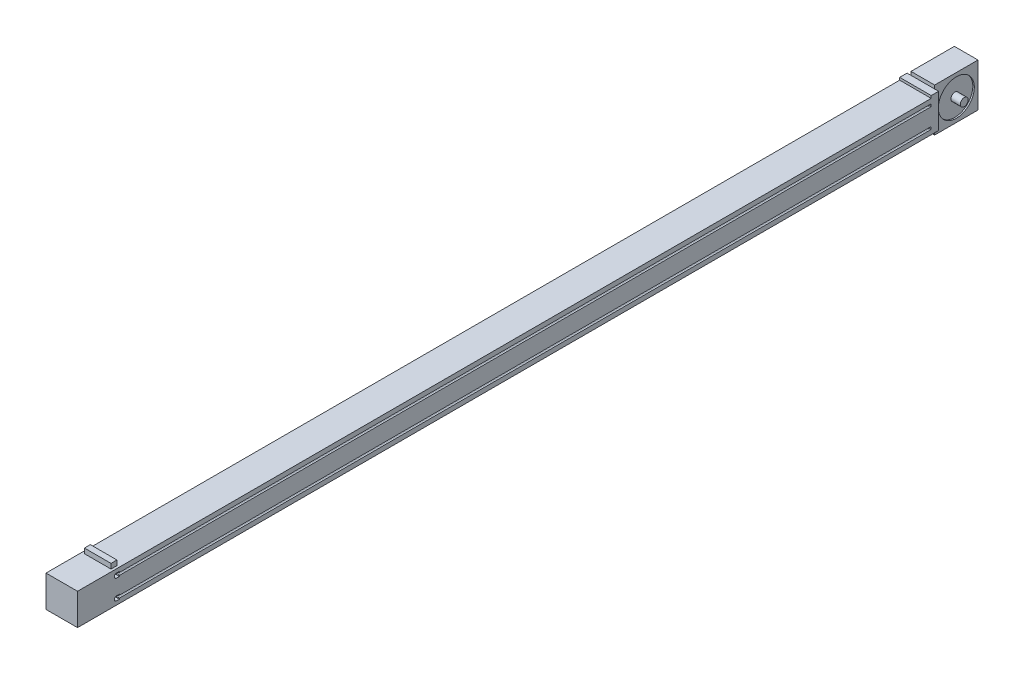
from build123d import *

# Parameters (mm, degrees)
EXTRUDE_642_DEPTH   = 1648
SKETCH_2_W          = 64
SKETCH_2_H          = 64
EXTRUDE_1_DEPTH     = 85
SKETCH_4_W          = 54
SKETCH_4_H          = 12
EXTRUDE_2_DEPTH     = 10
CUT_EXTRUDE_1_DEPTH = 10
SKETCH_6_W          = 64
SKETCH_6_H          = 69
EXTRUDE_3_DEPTH     = 15
SKETCH_7_W          = 48
SKETCH_7_H          = 88
EXTRUDE_4_DEPTH     = 88
SKETCH_8_R          = 36.5
CUT_EXTRUDE_2_DEPTH = 3
SKETCH_9_R          = 8
EXTRUDE_5_DEPTH     = 19


with BuildPart() as part:
    # 草图1 → Extrude 642 (new body)
    with BuildSketch(Plane.XY):
        Polygon((9.931917842, 6.925864063), (9.931917842, 41.925864063), (12.931917842, 41.925864063), (12.931917842, 40.425864063), (16.931917842, 40.425864063), (16.931917842, 48.425864063), (12.931917842, 48.425864063), (12.931917842, 46.925864063), (9.931917842, 46.925864063), (9.931917842, 56.425864063), (73.931917842, 56.425864063), (73.931917842, 46.925864063), (70.931917842, 46.925864063), (70.931917842, 48.425864063), (66.931917842, 48.425864063), (66.931917842, 40.425864063), (70.931917842, 40.425864063), (70.931917842, 41.925864063), (73.931917842, 41.925864063), (73.931917842, 6.925864063), (70.931917842, 6.925864063), (70.931917842, 8.425864063), (66.931917842, 8.425864063), (66.931917842, 0.425864063), (70.931917842, 0.425864063), (70.931917842, 1.925864063), (73.931917842, 1.925864063), (73.931917842, -7.574135937), (9.931917842, -7.574135937), (9.931917842, 1.925864063), (12.931917842, 1.925864063), (12.931917842, 0.425864063), (16.931917842, 0.425864063), (16.931917842, 8.425864063), (12.931917842, 8.425864063), (12.931917842, 6.925864063), align=None)
    extrude(amount=-EXTRUDE_642_DEPTH)

    # 草图2 → 凸台-拉伸1 (add)
    with BuildSketch(Plane.XY):
        with Locations((41.931917842, 24.425864063)):
            Rectangle(SKETCH_2_W, SKETCH_2_H)
    extrude(amount=EXTRUDE_1_DEPTH)

    # 草图4 → 凸台-拉伸2 (add)
    with BuildSketch(Plane(origin=(0, 56.425864063, 0), x_dir=(-1, 0, 0), z_dir=(0, 1, 0))):
        with Locations((-41.931917842, 6)):
            Rectangle(SKETCH_4_W, SKETCH_4_H)
    extrude(amount=EXTRUDE_2_DEPTH)

    # 草图5 → 切除-拉伸1 (cut)
    with BuildSketch(Plane(origin=(73.931917842, 0, 0), x_dir=(0, 0, -1), z_dir=(1, 0, 0))):
        with BuildLine():
            Line((0, 48.925864063), (-6, 48.925864063))
            ThreePointArc((-6, 48.925864063), (-8.828427125, 47.754291188), (-10, 44.925864063))
            Line((-10, 44.925864063), (-10, 43.925864063))
            ThreePointArc((-10, 43.925864063), (-8.828427125, 41.097436938), (-6, 39.925864063))
            Line((-6, 39.925864063), (0, 39.925864063))
            Line((0, 39.925864063), (0, 48.925864063))
        make_face()
        with BuildLine():
            Line((0, 8.925864063), (-6, 8.925864063))
            ThreePointArc((-6, 8.925864063), (-8.828427125, 7.754291188), (-10, 4.925864063))
            Line((-10, 4.925864063), (-10, 3.925864063))
            ThreePointArc((-10, 3.925864063), (-8.828427125, 1.097436938), (-6, -0.074135937))
            Line((-6, -0.074135937), (0, -0.074135937))
            Line((0, -0.074135937), (0, 8.925864063))
        make_face()
    cut_extrude_1 = extrude(amount=-CUT_EXTRUDE_1_DEPTH, mode=Mode.SUBTRACT)

    # 镜向1: 切除-拉伸1 across plane
    add(cut_extrude_1.mirror(Plane.ZY.offset(-41.931917842)), mode=Mode.SUBTRACT)

    # 草图6 → 凸台-拉伸3 (add)
    with BuildSketch(Plane(origin=(0, 0, -1648), x_dir=(-1, 0, 0), z_dir=(0, 0, -1))):
        with Locations((-41.931917842, 26.925864063)):
            Rectangle(SKETCH_6_W, SKETCH_6_H)
    extrude(amount=EXTRUDE_3_DEPTH)

    # 草图7 → 凸台-拉伸4 (add)
    with BuildSketch(Plane(origin=(0, 0, -1663), x_dir=(-1, 0, 0), z_dir=(0, 0, -1))):
        with Locations((-41.931917842, 24.425864063)):
            Rectangle(SKETCH_7_W, SKETCH_7_H)
    extrude(amount=EXTRUDE_4_DEPTH)

    # 草图8 → 切除-拉伸2 (cut)
    with BuildSketch(Plane.ZY.offset(-17.931917842)):
        with Locations((-1707, 24.425864063)):
            Circle(SKETCH_8_R)
    cut_extrude_2 = extrude(amount=-CUT_EXTRUDE_2_DEPTH, mode=Mode.SUBTRACT)

    # 草图9 → 凸台-拉伸5 (add)
    with BuildSketch(Plane.ZY.offset(-20.931917842)):
        with Locations((-1707, 24.425864063)):
            Circle(SKETCH_9_R)
    extrude_5 = extrude(amount=EXTRUDE_5_DEPTH)

    # 镜向2: 切除-拉伸2, 凸台-拉伸5 across plane
    add(cut_extrude_2.mirror(Plane.ZY.offset(-41.931917842)), mode=Mode.SUBTRACT)
    add(extrude_5.mirror(Plane.ZY.offset(-41.931917842)))


solid = part.part
